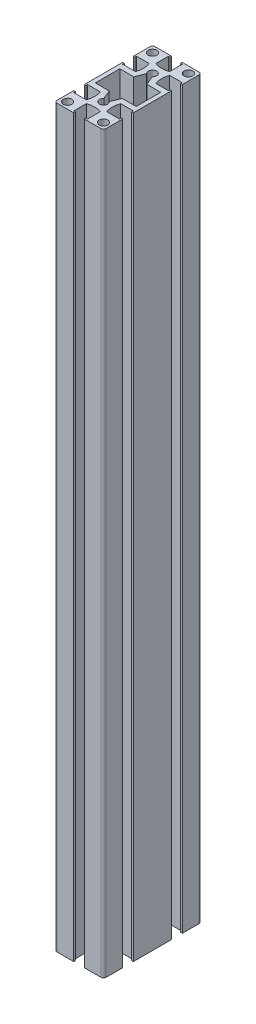
from build123d import *

# Parameters (mm, degrees)
SKETCH1_R                 = 2.65
F_30_X_60G_X_R1_5_1_DEPTH = 450


with BuildPart() as part:
    # Sketch1 → 工业铝型材 30 X 60G X R1.5(1) (new body)
    with BuildSketch(Plane(origin=(0, 0, 0), x_dir=(-1, 0, 0), z_dir=(0, 1, 0))):
        with BuildLine():
            Line((-3.25, 30), (-3.25, 29))
            Line((-3.25, 29), (-4.25, 29))
            Line((-4.25, 29), (-4.25, 21.277812156))
            ThreePointArc((-4.25, 21.277812156), (0, 20.5), (4.25, 21.277812156))
            Line((4.25, 21.277812156), (4.25, 29))
            Line((4.25, 29), (3.25, 29))
            Line((3.25, 29), (3.25, 30))
            Line((3.25, 30), (13.5, 30))
            ThreePointArc((13.5, 30), (14.560660172, 29.560660172), (15, 28.5))
            Line((15, 28.5), (15, 18.25))
            Line((15, 18.25), (14, 18.25))
            Line((14, 18.25), (14, 19.25))
            Line((14, 19.25), (6.277812156, 19.25))
            ThreePointArc((6.277812156, 19.25), (5.5, 15), (6.277812156, 10.75))
            Line((6.277812156, 10.75), (14, 10.75))
            Line((14, 10.75), (14, 11.75))
            Line((14, 11.75), (15, 11.75))
            Line((15, 11.75), (15, -11.75))
            Line((15, -11.75), (14, -11.75))
            Line((14, -11.75), (14, -10.75))
            Line((14, -10.75), (6.277812156, -10.75))
            ThreePointArc((6.277812156, -10.75), (5.5, -15), (6.277812156, -19.25))
            Line((6.277812156, -19.25), (14, -19.25))
            Line((14, -19.25), (14, -18.25))
            Line((14, -18.25), (15, -18.25))
            Line((15, -18.25), (15, -28.5))
            ThreePointArc((15, -28.5), (14.560660172, -29.560660172), (13.5, -30))
            Line((13.5, -30), (3.25, -30))
            Line((3.25, -30), (3.25, -29))
            Line((3.25, -29), (4.25, -29))
            Line((4.25, -29), (4.25, -21.277812156))
            ThreePointArc((4.25, -21.277812156), (0, -20.5), (-4.25, -21.277812156))
            Line((-4.25, -21.277812156), (-4.25, -29))
            Line((-4.25, -29), (-3.25, -29))
            Line((-3.25, -29), (-3.25, -30))
            Line((-3.25, -30), (-13.5, -30))
            ThreePointArc((-13.5, -30), (-14.560660172, -29.560660172), (-15, -28.5))
            Line((-15, -28.5), (-15, -18.25))
            Line((-15, -18.25), (-14, -18.25))
            Line((-14, -18.25), (-14, -19.25))
            Line((-14, -19.25), (-6.277812156, -19.25))
            ThreePointArc((-6.277812156, -19.25), (-5.5, -15), (-6.277812156, -10.75))
            Line((-6.277812156, -10.75), (-14, -10.75))
            Line((-14, -10.75), (-14, -11.75))
            Line((-14, -11.75), (-15, -11.75))
            Line((-15, -11.75), (-15, 11.75))
            Line((-15, 11.75), (-14, 11.75))
            Line((-14, 11.75), (-14, 10.75))
            Line((-14, 10.75), (-6.277812156, 10.75))
            ThreePointArc((-6.277812156, 10.75), (-5.5, 15), (-6.277812156, 19.25))
            Line((-6.277812156, 19.25), (-14, 19.25))
            Line((-14, 19.25), (-14, 18.25))
            Line((-14, 18.25), (-15, 18.25))
            Line((-15, 18.25), (-15, 28.5))
            ThreePointArc((-15, 28.5), (-14.560660172, 29.560660172), (-13.5, 30))
            Line((-13.5, 30), (-3.25, 30))
        make_face()
        with Locations((-11, 26)):
            Circle(SKETCH1_R, mode=Mode.SUBTRACT)
        with Locations((11, 26)):
            Circle(SKETCH1_R, mode=Mode.SUBTRACT)
        with Locations((11, -26)):
            Circle(SKETCH1_R, mode=Mode.SUBTRACT)
        with Locations((-11, -26)):
            Circle(SKETCH1_R, mode=Mode.SUBTRACT)
        with BuildLine():
            Line((-12.5, 7.5), (-4, 7.5))
            Line((-4, 7.5), (-1.665625283, 13.135679101))
            ThreePointArc((-1.665625283, 13.135679101), (0, 17.5), (1.665625283, 13.135679101))
            Line((1.665625283, 13.135679101), (4, 7.5))
            Line((4, 7.5), (12.5, 7.5))
            Line((12.5, 7.5), (12.5, -7.5))
            Line((12.5, -7.5), (4, -7.5))
            Line((4, -7.5), (1.665625283, -13.135679101))
            ThreePointArc((1.665625283, -13.135679101), (0, -17.5), (-1.665625283, -13.135679101))
            Line((-1.665625283, -13.135679101), (-4, -7.5))
            Line((-4, -7.5), (-12.5, -7.5))
            Line((-12.5, -7.5), (-12.5, 7.5))
        make_face(mode=Mode.SUBTRACT)
    extrude(amount=F_30_X_60G_X_R1_5_1_DEPTH)


solid = part.part
